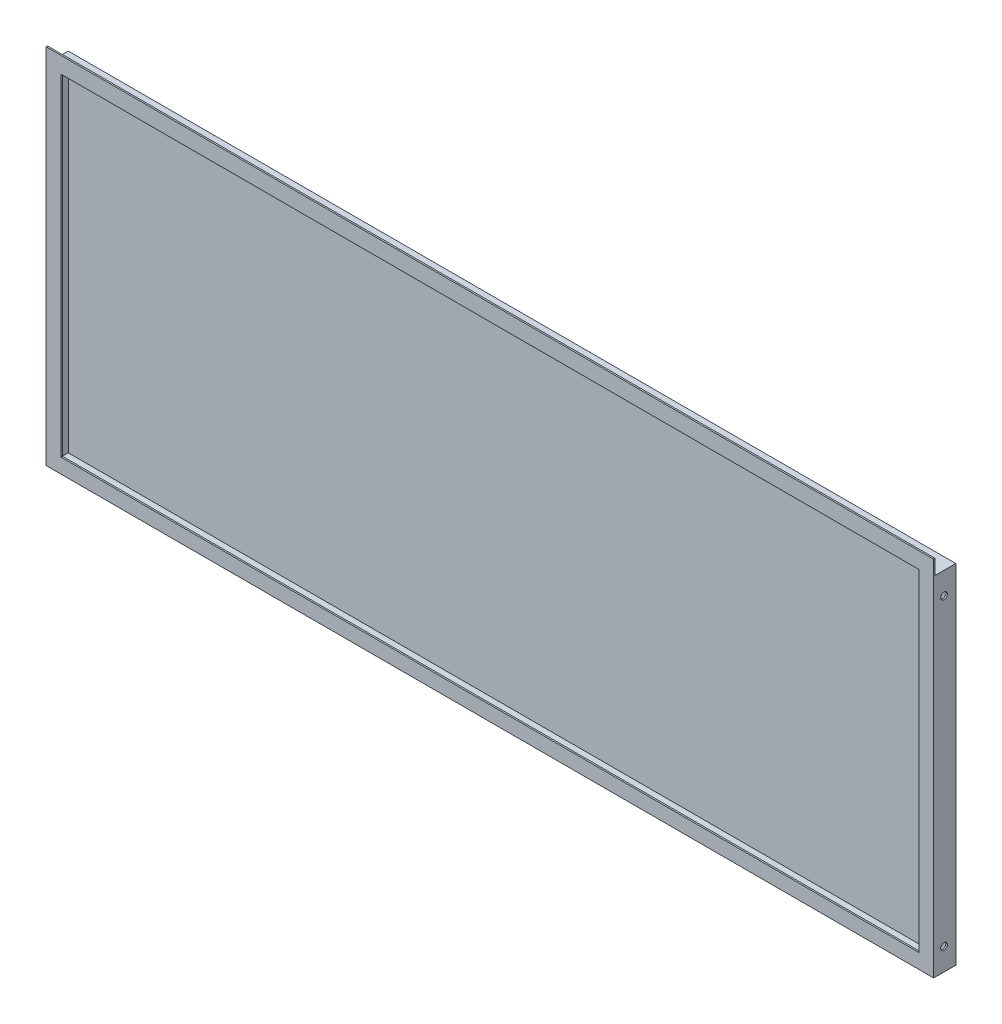
SolidWorks part; units mm, degrees
ref_plane "前视基准面" through (0, 0, 0) normal (0, 0, 1) x (1, 0, 0)
ref_plane "上视基准面" through (0, 0, 0) normal (0, 1, 0) x (1, 0, 0)
ref_plane "右视基准面" through (0, 0, 0) normal (1, 0, 0) x (0, 0, -1)
sketch "草图1" plane through (0, 0, 0) normal (0, 0, 1) x (1, 0, 0)
  line L1 (0, 0) -> (1204, 0)
  line L2 (0, 0) -> (0, 472)
  line L3 (0, 472) -> (1204, 472)
  line L4 (1204, 0) -> (1204, 472)
  dimension "D1" = 472
  dimension "D2" = 1204
extrude "凸台-拉伸1" add sketch "草图1" along normal blind 30
shell "抽壳1" thickness 2
sketch "草图2" plane through (0, 0, 30) normal (0, 0, 1) x (1, 0, 0)
  line L0 (1202, 470) -> (2, 470) construction
  line L1 (0, 492) -> (1204, 492)
  line L2 (0, 492) -> (0, 0)
  line L3 (0, 0) -> (1204, 0)
  line L4 (1204, 492) -> (1204, 0)
  line L5 (0, 472) -> (0, 0) construction
  line L6 (1204, 472) -> (0, 472) construction
  line L7 (1202, 470) -> (2, 470) construction
  line L8 (20, 20) -> (1184, 20)
  line L9 (20, 20) -> (20, 470)
  line L10 (20, 470) -> (1184, 470)
  line L11 (1184, 20) -> (1184, 470)
  dimension "D1" = 20
  dimension "D2" = 20
  dimension "D3" = 20
  dimension "D4" = 20
extrude "凸台-拉伸2" add sketch "草图2" against normal blind 2
sketch "草图3" plane through (2, 0, 0) normal (1, 0, 0) x (0, 0, -1)
  line L0 (-16, 470) -> (-16, -9.9646) construction
  line L1 (-28, 470) -> (-2, 470) construction
  line L2 (-30, 0) -> (-30, 492) construction
  line L3 (-30, 0) -> (0, 0) construction
  line L4 (-28, 472) -> (0, 472) construction
  circle A0 centre (-16, 442) radius 4.5
  circle A1 centre (-16, 30) radius 4.5
  dimension "D2" = 9
  dimension "D3" = 9
  dimension "D4" = 30
  dimension "D5" = 30
  dimension "D1" = 14
extrude "切除-拉伸1" cut sketch "草图3" against normal blind 72 and the other way blind 1295
sketch "草图4" plane through (0, 2, 0) normal (0, 1, 0) x (1, 0, 0)
  line L0 (1202, -16) -> (-111.2408, -16) construction
  line L1 (1202, -28) -> (1202, -2) construction
  line L2 (0, -30) -> (1204, -30) construction
  line L3 (1204, -30) -> (1204, 0) construction
  line L4 (0, -30) -> (0, 0) construction
  circle A0 centre (1174, -16) radius 4.5
  circle A1 centre (30, -16) radius 4.5
  circle A2 centre (1065, -16) radius 4.5
  circle A3 centre (965, -16) radius 4.5
  circle A4 centre (500, -16) radius 4.5
  dimension "D2" = 9
  dimension "D3" = 30
  dimension "D4" = 9
  dimension "D5" = 30
  dimension "D6" = 9
  dimension "D7" = 139
  dimension "D8" = 9
  dimension "D9" = 935
  dimension "D10" = 9
  dimension "D11" = 470
  dimension "D1" = 14
extrude "切除-拉伸2" cut sketch "草图4" against normal blind 45
